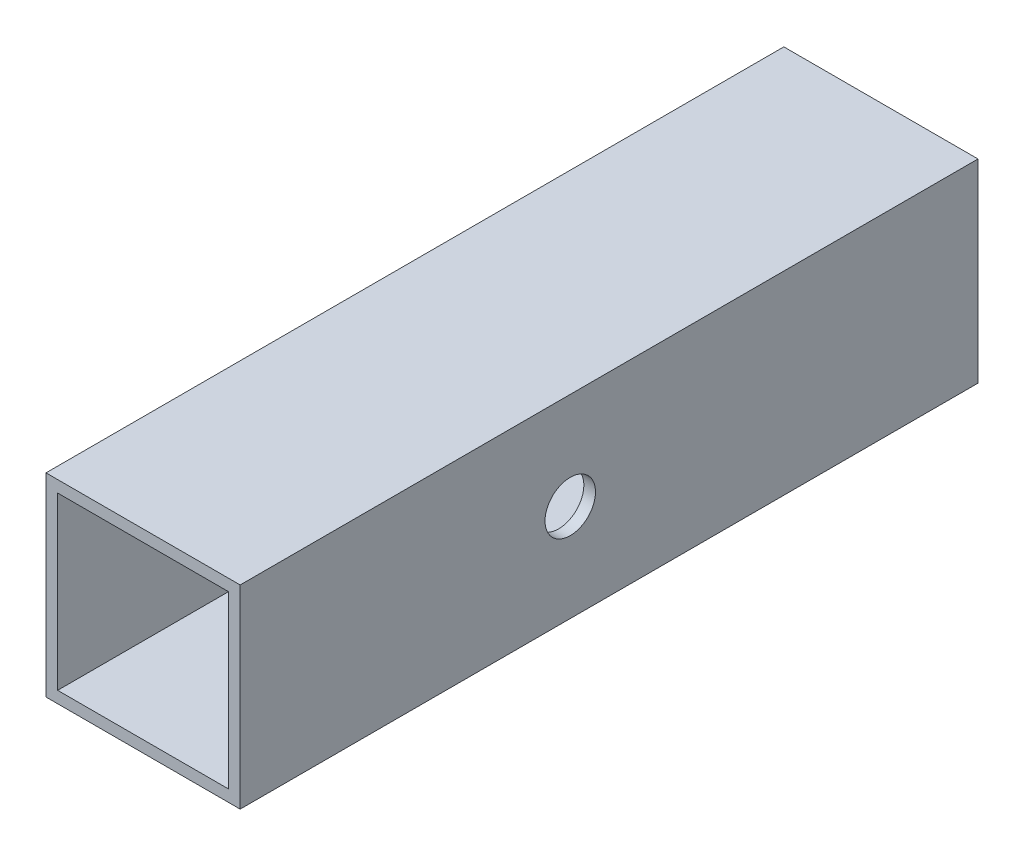
from build123d import *

# Parameters (mm, degrees)
SKETCH_1_W          = 50
SKETCH_1_H          = 50
SKETCH_1_W_2        = 44
SKETCH_1_H_2        = 44
EXTRUDE_2_DEPTH     = 190
SKETCH_5_R          = 6.5
CUT_EXTRUDE_1_DEPTH = 130


with BuildPart() as part:
    # 草图1 → 凸台-拉伸2 (new body)
    with BuildSketch(Plane.XY):
        with Locations((25, -25)):
            Rectangle(SKETCH_1_W, SKETCH_1_H)
        with Locations((25, -25)):
            Rectangle(SKETCH_1_W_2, SKETCH_1_H_2, mode=Mode.SUBTRACT)
    extrude(amount=EXTRUDE_2_DEPTH)

    # 草图5 → 切除-拉伸1 (cut)
    with BuildSketch(Plane(origin=(50, 0, 0), x_dir=(0, 0, -1), z_dir=(1, 0, 0))):
        with Locations(Location((-105, -25, 0), (0, 0, 90))):
            Circle(SKETCH_5_R)
        with Locations((-324.839370649, -25)):
            Circle(SKETCH_5_R)
    extrude(amount=-CUT_EXTRUDE_1_DEPTH, mode=Mode.SUBTRACT)


solid = part.part
